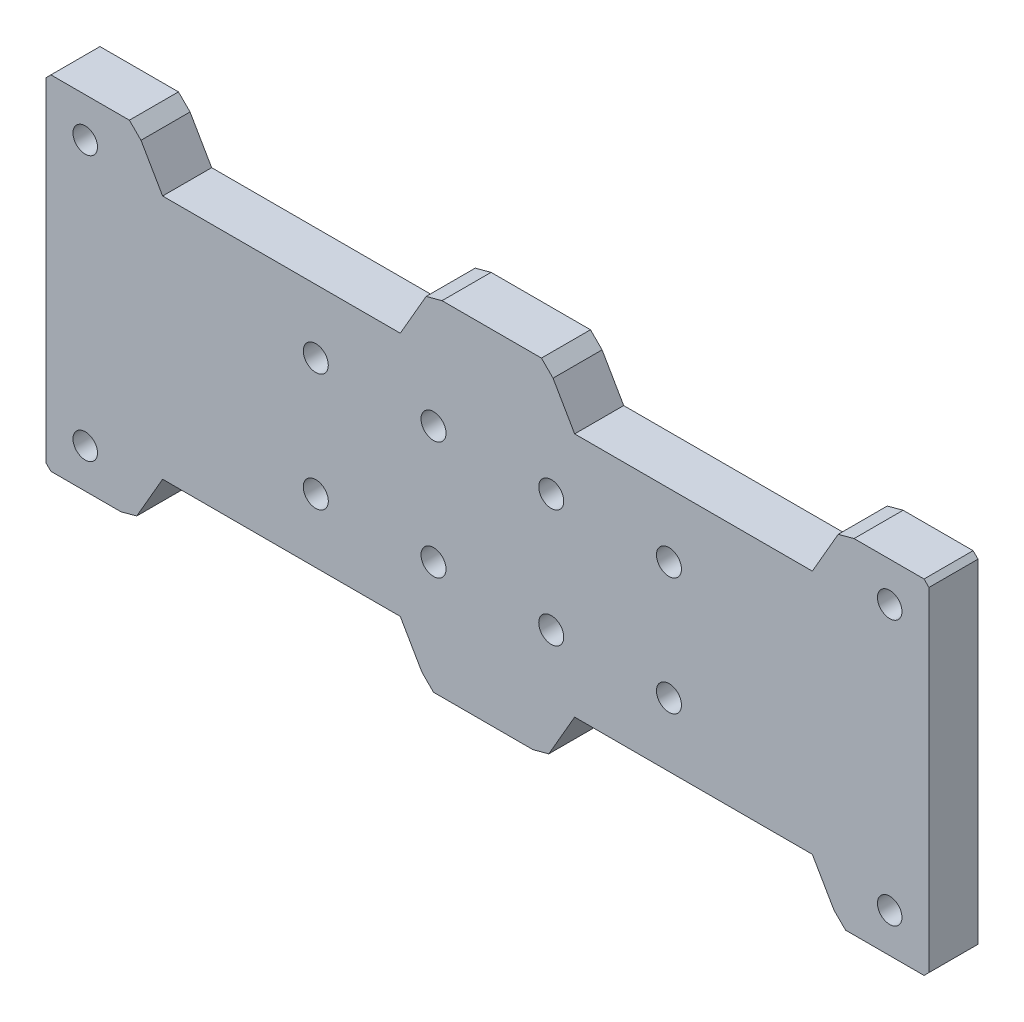
SolidWorks part; units mm, degrees
ref_plane "Front Plane" through (0, 0, 0) normal (0, 0, 1) x (1, 0, 0)
ref_plane "Top Plane" through (0, 0, 0) normal (0, 1, 0) x (1, 0, 0)
ref_plane "Right Plane" through (0, 0, 0) normal (1, 0, 0) x (0, 0, -1)
other "Configuration Table"
sketch "Sketch1" plane through (0, 0, 0) normal (0, 0, 1) x (1, 0, 0)
  line L1 (-90, 35) -> (90, 35)
  line L2 (-90, 35) -> (-90, -35)
  line L3 (-90, -35) -> (90, -35)
  line L4 (90, 35) -> (90, -35)
  line L5 (-90, 35) -> (90, -35) construction
  line L6 (-90, -35) -> (90, 35) construction
  point P0 (0, 0)
  dimension "D1" = 180
  dimension "D2" = 70
extrude "Boss-Extrude1" add sketch "Sketch1" along normal blind 10
sketch "Sketch2" plane through (0, 0, 10) normal (0, 0, 1) x (1, 0, 0)
  line L0 (0, 0) -> (0, 35) construction
  line L1 (90, 35) -> (-90, 35) construction
  line L2 (-90, 0) -> (90, 0) construction
  line L3 (-90, 35) -> (-90, -35) construction
  line L4 (90, -35) -> (90, 35) construction
  line L5 (-72, 35) -> (-66.2265, 25)
  line L6 (-66.2265, 25) -> (-17.7735, 25)
  line L7 (-17.7735, 25) -> (-12, 35)
  line L8 (-72, 35) -> (-12, 35)
  line L9 (72, 35) -> (12, 35)
  line L10 (17.7735, 25) -> (12, 35)
  line L11 (66.2265, 25) -> (17.7735, 25)
  line L12 (72, 35) -> (66.2265, 25)
  line L13 (72, -35) -> (66.2265, -25)
  line L14 (66.2265, -25) -> (17.7735, -25)
  line L15 (17.7735, -25) -> (12, -35)
  line L16 (72, -35) -> (12, -35)
  line L17 (-72, -35) -> (-12, -35)
  line L18 (-17.7735, -25) -> (-12, -35)
  line L19 (-66.2265, -25) -> (-17.7735, -25)
  line L20 (-72, -35) -> (-66.2265, -25)
  dimension "D1" = 120
  dimension "D2" = 120
  dimension "D3" = 60
  dimension "D4" = 12
  dimension "D5" = 10
extrude "Cut-Extrude1" cut sketch "Sketch2" against normal through all
sketch "Sketch3" plane through (0, 0, 10) normal (0, 0, 1) x (1, 0, 0)
  line L0 (0, 0) -> (0, 35) construction
  line L1 (12, 35) -> (-12, 35) construction
  line L2 (0, 0) -> (-90, 0) construction
  line L3 (-90, 35) -> (-90, -35) construction
  line L4 (-72, 35) -> (-90, 35) construction
  circle A0 centre (-82, 27) radius 2.5
  circle A1 centre (82, 27) radius 2.5
  circle A2 centre (82, -27) radius 2.5
  circle A3 centre (-82, -27) radius 2.5
  dimension "D1" = 5
  dimension "D2" = 8
  dimension "D3" = 8
extrude "Cut-Extrude2" cut sketch "Sketch3" against normal through all
chamfer "Chamfer1" distance 1 angle 45 12 edges at (-90, 35, 5) (-72, 35, 5) (-12, 35, 5) (12, 35, 5) (72, 35, 5) (90, 35, 5) (90, -35, 5) (72, -35, 5) (12, -35, 5) (-12, -35, 5) (-72, -35, 5) (-90, -35, 5)
sketch "Sketch4" plane through (0, 0, 10) normal (0, 0, 1) x (1, 0, 0)
  line L0 (0, 0) -> (0, 35) construction
  line L3 (11, 35) -> (-9.2679, 35) construction
  line L4 (0, 0) -> (-90, 0) construction
  line L5 (-90, 34) -> (-90, -34) construction
  circle A0 centre (-35, 12) radius 2.55
  circle A1 centre (-11, 12) radius 2.55
  circle A2 centre (13, 12) radius 2.55
  circle A3 centre (37, 12) radius 2.55
  circle A4 centre (37, -12) radius 2.55
  circle A5 centre (13, -12) radius 2.55
  circle A6 centre (-11, -12) radius 2.55
  circle A7 centre (-35, -12) radius 2.55
  dimension "D1" = 5.1
  dimension "D2" = 12
  dimension "D3" = 35
  dimension "D4" = 4
extrude "Cut-Extrude3" cut sketch "Sketch4" against normal through all
